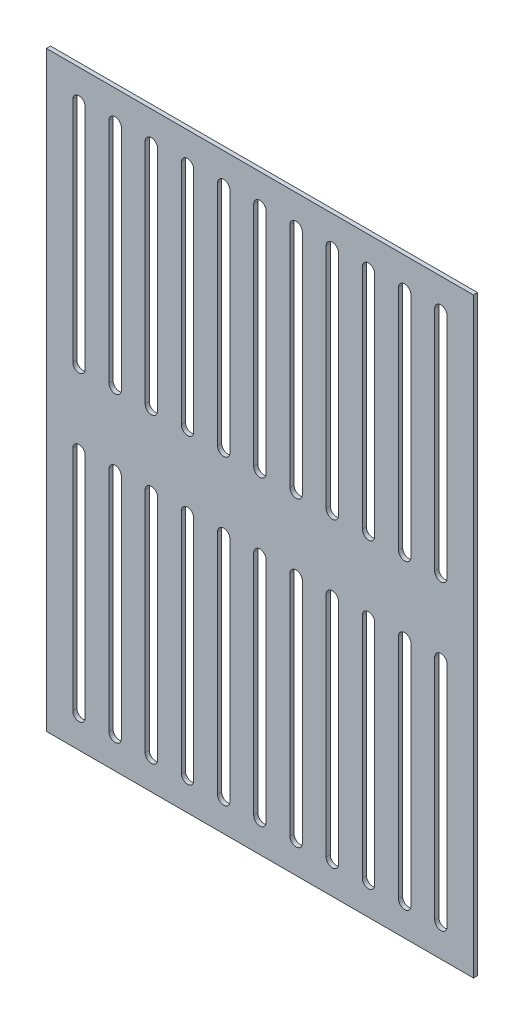
SolidWorks part; units mm, degrees
material "304 钣金"
ref_plane "Front plane" through (0, 0, 0) normal (0, 0, 1) x (1, 0, 0)
ref_plane "Top plane" through (0, 0, 0) normal (0, 1, 0) x (1, 0, 0)
ref_plane "Right plane" through (0, 0, 0) normal (1, 0, 0) x (0, 0, -1)
sketch "Sketch1" plane through (0, 0, 0) normal (0, 0, 1) x (1, 0, 0)
  line L1 (206.5, 286) -> (-206.5, 286)
  line L2 (206.5, 286) -> (206.5, -286)
  line L3 (206.5, -286) -> (-206.5, -286)
  line L4 (-206.5, 286) -> (-206.5, -286)
  line L5 (206.5, 286) -> (-206.5, -286) construction
  line L6 (206.5, -286) -> (-206.5, 286) construction
  point P0 (0, 0)
  dimension "D1" = 413
  dimension "D2" = 572
extrude "Boss-Extrude1" add sketch "Sketch1" along normal blind 4
sketch "Sketch2" plane through (0, 0, 4) normal (0, 0, 1) x (1, 0, 0)
  line L0 (0, -233.0002) -> (0, 233.0002) construction
  line L1 (0, 0) -> (277.4997, 0) construction
  line L2 (0, 256) -> (0, 36) construction
  line L3 (6, 256) -> (6, 36)
  line L4 (-6, 256) -> (-6, 36)
  line L5 (206.5, 286) -> (-206.5, 286) construction
  line L6 (35, 256) -> (35, 36) construction
  line L7 (41, 256) -> (41, 36)
  line L8 (29, 256) -> (29, 36)
  line L9 (70, 256) -> (70, 36) construction
  line L10 (76, 256) -> (76, 36)
  line L11 (64, 256) -> (64, 36)
  line L12 (105, 256) -> (105, 36) construction
  line L13 (111, 256) -> (111, 36)
  line L14 (99, 256) -> (99, 36)
  line L15 (140, 256) -> (140, 36) construction
  line L16 (146, 256) -> (146, 36)
  line L17 (134, 256) -> (134, 36)
  line L18 (175, 256) -> (175, 36) construction
  line L19 (181, 256) -> (181, 36)
  line L20 (169, 256) -> (169, 36)
  line L21 (-175, 256) -> (-175, 36) construction
  line L22 (-181, 256) -> (-181, 36)
  line L23 (-169, 256) -> (-169, 36)
  line L24 (-140, 256) -> (-140, 36) construction
  line L25 (-146, 256) -> (-146, 36)
  line L26 (-134, 256) -> (-134, 36)
  line L27 (-105, 256) -> (-105, 36) construction
  line L28 (-111, 256) -> (-111, 36)
  line L29 (-99, 256) -> (-99, 36)
  line L30 (-70, 256) -> (-70, 36) construction
  line L31 (-76, 256) -> (-76, 36)
  line L32 (-64, 256) -> (-64, 36)
  line L33 (-35, 256) -> (-35, 36) construction
  line L34 (-41, 256) -> (-41, 36)
  line L35 (-29, 256) -> (-29, 36)
  line L36 (-35, 256) -> (-35, 36) construction
  line L37 (-41, 256) -> (-41, 36)
  line L38 (-29, 256) -> (-29, 36)
  line L39 (-70, 256) -> (-70, 36) construction
  line L40 (-76, 256) -> (-76, 36)
  line L41 (-64, 256) -> (-64, 36)
  line L42 (-105, 256) -> (-105, 36) construction
  line L43 (-111, 256) -> (-111, 36)
  line L44 (-99, 256) -> (-99, 36)
  line L45 (-140, 256) -> (-140, 36) construction
  line L46 (-146, 256) -> (-146, 36)
  line L47 (-134, 256) -> (-134, 36)
  line L48 (-175, 256) -> (-175, 36) construction
  line L49 (-181, 256) -> (-181, 36)
  line L50 (-169, 256) -> (-169, 36)
  line L51 (175, 256) -> (175, 36) construction
  line L52 (181, 256) -> (181, 36)
  line L53 (169, 256) -> (169, 36)
  line L54 (140, 256) -> (140, 36) construction
  line L55 (146, 256) -> (146, 36)
  line L56 (134, 256) -> (134, 36)
  line L57 (105, 256) -> (105, 36) construction
  line L58 (111, 256) -> (111, 36)
  line L59 (99, 256) -> (99, 36)
  line L60 (70, 256) -> (70, 36) construction
  line L61 (76, 256) -> (76, 36)
  line L62 (64, 256) -> (64, 36)
  line L63 (35, 256) -> (35, 36) construction
  line L64 (41, 256) -> (41, 36)
  line L65 (29, 256) -> (29, 36)
  line L66 (-35, -256) -> (-35, -36) construction
  line L67 (-41, -256) -> (-41, -36)
  line L68 (-29, -256) -> (-29, -36)
  line L69 (-70, -256) -> (-70, -36) construction
  line L70 (-76, -256) -> (-76, -36)
  line L71 (-64, -256) -> (-64, -36)
  line L72 (-105, -256) -> (-105, -36) construction
  line L73 (-111, -256) -> (-111, -36)
  line L74 (-99, -256) -> (-99, -36)
  line L75 (-140, -256) -> (-140, -36) construction
  line L76 (-146, -256) -> (-146, -36)
  line L77 (-134, -256) -> (-134, -36)
  line L78 (-175, -256) -> (-175, -36) construction
  line L79 (-181, -256) -> (-181, -36)
  line L80 (-169, -256) -> (-169, -36)
  line L81 (175, -256) -> (175, -36) construction
  line L82 (181, -256) -> (181, -36)
  line L83 (169, -256) -> (169, -36)
  line L84 (140, -256) -> (140, -36) construction
  line L85 (146, -256) -> (146, -36)
  line L86 (134, -256) -> (134, -36)
  line L87 (105, -256) -> (105, -36) construction
  line L88 (111, -256) -> (111, -36)
  line L89 (99, -256) -> (99, -36)
  line L90 (70, -256) -> (70, -36) construction
  line L91 (76, -256) -> (76, -36)
  line L92 (64, -256) -> (64, -36)
  line L93 (35, -256) -> (35, -36) construction
  line L94 (41, -256) -> (41, -36)
  line L95 (29, -256) -> (29, -36)
  line L96 (-35, -256) -> (-35, -36) construction
  line L97 (-41, -256) -> (-41, -36)
  line L98 (-29, -256) -> (-29, -36)
  line L99 (-70, -256) -> (-70, -36) construction
  line L100 (-76, -256) -> (-76, -36)
  line L101 (-64, -256) -> (-64, -36)
  line L102 (-105, -256) -> (-105, -36) construction
  line L103 (-111, -256) -> (-111, -36)
  line L104 (-99, -256) -> (-99, -36)
  line L105 (-140, -256) -> (-140, -36) construction
  line L106 (-146, -256) -> (-146, -36)
  line L107 (-134, -256) -> (-134, -36)
  line L108 (-175, -256) -> (-175, -36) construction
  line L109 (-181, -256) -> (-181, -36)
  line L110 (-169, -256) -> (-169, -36)
  line L111 (175, -256) -> (175, -36) construction
  line L112 (181, -256) -> (181, -36)
  line L113 (169, -256) -> (169, -36)
  line L114 (140, -256) -> (140, -36) construction
  line L115 (146, -256) -> (146, -36)
  line L116 (134, -256) -> (134, -36)
  line L117 (105, -256) -> (105, -36) construction
  line L118 (111, -256) -> (111, -36)
  line L119 (99, -256) -> (99, -36)
  line L120 (70, -256) -> (70, -36) construction
  line L121 (76, -256) -> (76, -36)
  line L122 (64, -256) -> (64, -36)
  line L123 (35, -256) -> (35, -36) construction
  line L124 (41, -256) -> (41, -36)
  line L125 (29, -256) -> (29, -36)
  line L126 (0, -256) -> (0, -36) construction
  line L127 (6, -256) -> (6, -36)
  line L128 (-6, -256) -> (-6, -36)
  arc A0 (6, 256) -> (-6, 256) centre (0, 256) ccw
  arc A1 (-6, 36) -> (6, 36) centre (0, 36) ccw
  arc A2 (41, 256) -> (29, 256) centre (35, 256) ccw
  arc A3 (29, 36) -> (41, 36) centre (35, 36) ccw
  arc A4 (76, 256) -> (64, 256) centre (70, 256) ccw
  arc A5 (64, 36) -> (76, 36) centre (70, 36) ccw
  arc A6 (111, 256) -> (99, 256) centre (105, 256) ccw
  arc A7 (99, 36) -> (111, 36) centre (105, 36) ccw
  arc A8 (146, 256) -> (134, 256) centre (140, 256) ccw
  arc A9 (134, 36) -> (146, 36) centre (140, 36) ccw
  arc A10 (181, 256) -> (169, 256) centre (175, 256) ccw
  arc A11 (169, 36) -> (181, 36) centre (175, 36) ccw
  arc A12 (-181, 256) -> (-169, 256) centre (-175, 256) cw
  arc A13 (-169, 36) -> (-181, 36) centre (-175, 36) cw
  arc A14 (-146, 256) -> (-134, 256) centre (-140, 256) cw
  arc A15 (-134, 36) -> (-146, 36) centre (-140, 36) cw
  arc A16 (-111, 256) -> (-99, 256) centre (-105, 256) cw
  arc A17 (-99, 36) -> (-111, 36) centre (-105, 36) cw
  arc A18 (-76, 256) -> (-64, 256) centre (-70, 256) cw
  arc A19 (-64, 36) -> (-76, 36) centre (-70, 36) cw
  arc A20 (-41, 256) -> (-29, 256) centre (-35, 256) cw
  arc A21 (-29, 36) -> (-41, 36) centre (-35, 36) cw
  arc A22 (-41, 256) -> (-29, 256) centre (-35, 256) cw
  arc A23 (-29, 36) -> (-41, 36) centre (-35, 36) cw
  arc A24 (-76, 256) -> (-64, 256) centre (-70, 256) cw
  arc A25 (-64, 36) -> (-76, 36) centre (-70, 36) cw
  arc A26 (-111, 256) -> (-99, 256) centre (-105, 256) cw
  arc A27 (-99, 36) -> (-111, 36) centre (-105, 36) cw
  arc A28 (-146, 256) -> (-134, 256) centre (-140, 256) cw
  arc A29 (-134, 36) -> (-146, 36) centre (-140, 36) cw
  arc A30 (-181, 256) -> (-169, 256) centre (-175, 256) cw
  arc A31 (-169, 36) -> (-181, 36) centre (-175, 36) cw
  arc A32 (181, 256) -> (169, 256) centre (175, 256) ccw
  arc A33 (169, 36) -> (181, 36) centre (175, 36) ccw
  arc A34 (146, 256) -> (134, 256) centre (140, 256) ccw
  arc A35 (134, 36) -> (146, 36) centre (140, 36) ccw
  arc A36 (111, 256) -> (99, 256) centre (105, 256) ccw
  arc A37 (99, 36) -> (111, 36) centre (105, 36) ccw
  arc A38 (76, 256) -> (64, 256) centre (70, 256) ccw
  arc A39 (64, 36) -> (76, 36) centre (70, 36) ccw
  arc A40 (41, 256) -> (29, 256) centre (35, 256) ccw
  arc A41 (29, 36) -> (41, 36) centre (35, 36) ccw
  arc A42 (-41, -256) -> (-29, -256) centre (-35, -256) ccw
  arc A43 (-29, -36) -> (-41, -36) centre (-35, -36) ccw
  arc A44 (-76, -256) -> (-64, -256) centre (-70, -256) ccw
  arc A45 (-64, -36) -> (-76, -36) centre (-70, -36) ccw
  arc A46 (-111, -256) -> (-99, -256) centre (-105, -256) ccw
  arc A47 (-99, -36) -> (-111, -36) centre (-105, -36) ccw
  arc A48 (-146, -256) -> (-134, -256) centre (-140, -256) ccw
  arc A49 (-134, -36) -> (-146, -36) centre (-140, -36) ccw
  arc A50 (-181, -256) -> (-169, -256) centre (-175, -256) ccw
  arc A51 (-169, -36) -> (-181, -36) centre (-175, -36) ccw
  arc A52 (181, -256) -> (169, -256) centre (175, -256) cw
  arc A53 (169, -36) -> (181, -36) centre (175, -36) cw
  arc A54 (146, -256) -> (134, -256) centre (140, -256) cw
  arc A55 (134, -36) -> (146, -36) centre (140, -36) cw
  arc A56 (111, -256) -> (99, -256) centre (105, -256) cw
  arc A57 (99, -36) -> (111, -36) centre (105, -36) cw
  arc A58 (76, -256) -> (64, -256) centre (70, -256) cw
  arc A59 (64, -36) -> (76, -36) centre (70, -36) cw
  arc A60 (41, -256) -> (29, -256) centre (35, -256) cw
  arc A61 (29, -36) -> (41, -36) centre (35, -36) cw
  arc A62 (-41, -256) -> (-29, -256) centre (-35, -256) ccw
  arc A63 (-29, -36) -> (-41, -36) centre (-35, -36) ccw
  arc A64 (-76, -256) -> (-64, -256) centre (-70, -256) ccw
  arc A65 (-64, -36) -> (-76, -36) centre (-70, -36) ccw
  arc A66 (-111, -256) -> (-99, -256) centre (-105, -256) ccw
  arc A67 (-99, -36) -> (-111, -36) centre (-105, -36) ccw
  arc A68 (-146, -256) -> (-134, -256) centre (-140, -256) ccw
  arc A69 (-134, -36) -> (-146, -36) centre (-140, -36) ccw
  arc A70 (-181, -256) -> (-169, -256) centre (-175, -256) ccw
  arc A71 (-169, -36) -> (-181, -36) centre (-175, -36) ccw
  arc A72 (181, -256) -> (169, -256) centre (175, -256) cw
  arc A73 (169, -36) -> (181, -36) centre (175, -36) cw
  arc A74 (146, -256) -> (134, -256) centre (140, -256) cw
  arc A75 (134, -36) -> (146, -36) centre (140, -36) cw
  arc A76 (111, -256) -> (99, -256) centre (105, -256) cw
  arc A77 (99, -36) -> (111, -36) centre (105, -36) cw
  arc A78 (76, -256) -> (64, -256) centre (70, -256) cw
  arc A79 (64, -36) -> (76, -36) centre (70, -36) cw
  arc A80 (41, -256) -> (29, -256) centre (35, -256) cw
  arc A81 (29, -36) -> (41, -36) centre (35, -36) cw
  arc A82 (6, -256) -> (-6, -256) centre (0, -256) cw
  arc A83 (-6, -36) -> (6, -36) centre (0, -36) cw
  point P6 (0, 146)
  point P17 (35, 146)
  point P24 (70, 146)
  point P31 (105, 146)
  point P38 (140, 146)
  point P45 (175, 146)
  point P50 (-175, 146)
  point P57 (-140, 146)
  point P64 (-105, 146)
  point P71 (-70, 146)
  point P78 (-35, 146)
  point P146 (-35, -146)
  point P153 (-70, -146)
  point P160 (-105, -146)
  point P167 (-140, -146)
  point P174 (-175, -146)
  point P181 (175, -146)
  point P188 (140, -146)
  point P195 (105, -146)
  point P202 (70, -146)
  point P209 (35, -146)
  point P276 (0, -146)
  dimension "D1" = 6
  dimension "D2" = 220
  dimension "D3" = 30
  dimension "D4" = 6
extrude "Cut-Extrude1" cut sketch "Sketch2" against normal blind 4 contours L74 A47 L73 A46 | L71 A45 L70 A44 | L68 A43 L67 A42 | A83 L128 A82 L127 | A61 L95 A60 L94 | A59 L92 A58 L91 | A53 L83 A52 L82 | A55 L86 A54 L85 | A57 L89 A56 L88 | A13 L23 A12 L22 | A15 L26 A14 L25 | A17 L29 A16 L28 | A19 L32 A18 L31 | A21 L35 A20 L34 | L4 A1 L3 A0 | L11 A5 L10 A4 | L14 A7 L13 A6 | L17 A9 L16 A8 | L20 A11 L19 A10 | L79 A51 L80 A50 | L76 A49 L77 A48 | L8 A3 L7 A2
